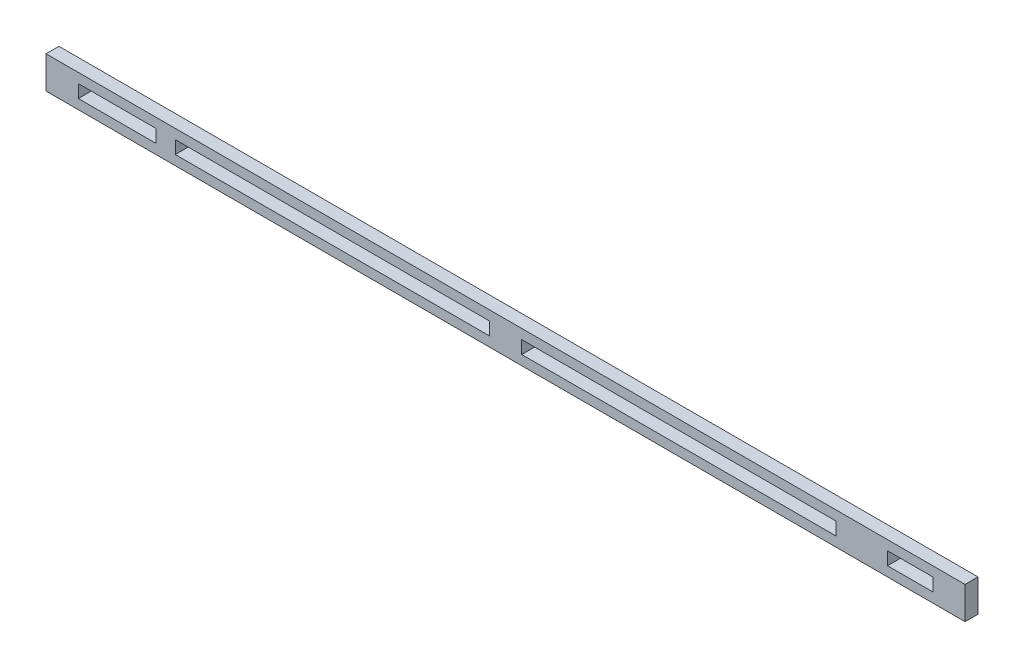
from build123d import *

# Parameters (mm, degrees)
SKETCH1_W           = 14220
SKETCH1_H           = 500
BOSS_EXTRUDE1_DEPTH = 200
SKETCH2_W           = 1200
SKETCH2_H           = 200
SKETCH2_W_2         = 4860
CUT_EXTRUDE1_DEPTH  = 7118.204507389
SKETCH4_W           = 500
SKETCH4_H           = 200
BOSS_EXTRUDE2_DEPTH = 200


with BuildPart() as part:
    # Sketch1 → Boss-Extrude1 (new body)
    with BuildSketch(Plane.XY):
        Rectangle(SKETCH1_W, SKETCH1_H)
    extrude(amount=BOSS_EXTRUDE1_DEPTH)

    # Sketch2 → Cut-Extrude1 (cut, through all)
    with BuildSketch(Plane.XY.offset(200)):
        with Locations((-6010, 0)):
            Rectangle(SKETCH2_W, SKETCH2_H)
        with Locations((-2680, 0)):
            Rectangle(SKETCH2_W_2, SKETCH2_H)
        with Locations((2680, 0)):
            Rectangle(SKETCH2_W_2, SKETCH2_H)
        with Locations((6010, 0)):
            Rectangle(SKETCH2_W, SKETCH2_H)
    extrude(amount=-CUT_EXTRUDE1_DEPTH, mode=Mode.SUBTRACT)

    # Sketch4 → Boss-Extrude2 (add)
    with BuildSketch(Plane.XY.offset(200)):
        with Locations((5660, 0)):
            Rectangle(SKETCH4_W, SKETCH4_H)
    extrude(amount=-BOSS_EXTRUDE2_DEPTH)


solid = part.part
